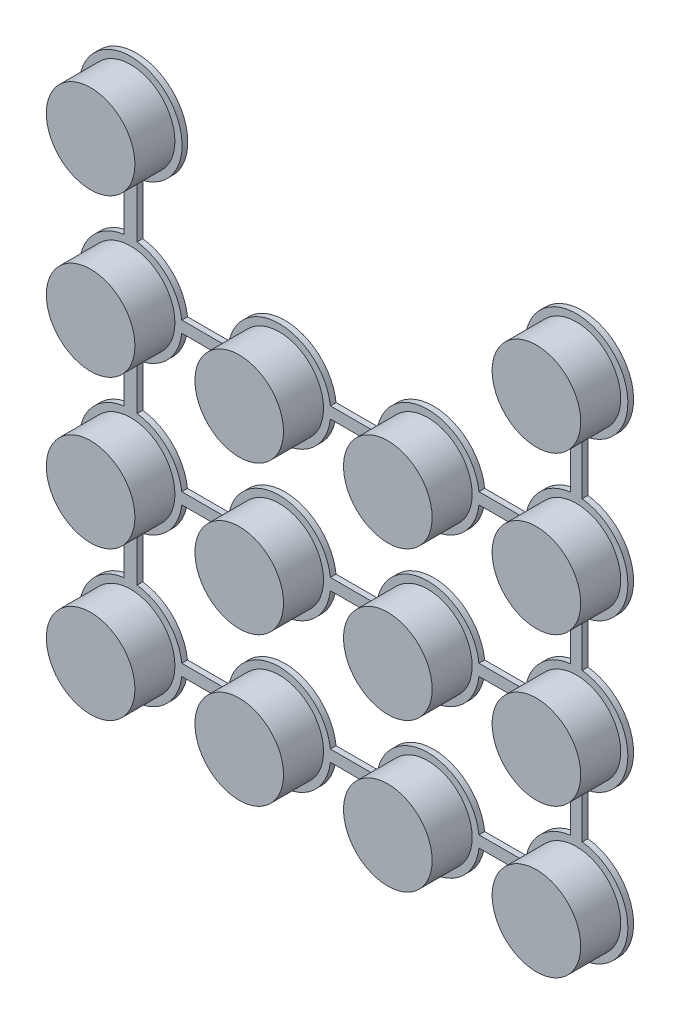
from build123d import *

# Parameters (mm, degrees)
BOSS_EXTRUDE1_DEPTH = 1
SKETCH2_R           = 7.75
BOSS_EXTRUDE2_DEPTH = 7


with BuildPart() as part:
    # Sketch1 → Boss-Extrude1 (new body)
    with BuildSketch(Plane.XY):
        with BuildLine():
            Line((-40.125, 93.570589325), (-40.125, 83.929410675))
            ThreePointArc((-40.125, 83.929410675), (-48, 75), (-40.125, 66.070589325))
            Line((-40.125, 66.070589325), (-40.125, 57.929410675))
            ThreePointArc((-40.125, 57.929410675), (-48, 49), (-40.125, 40.070589325))
            Line((-40.125, 40.070589325), (-40.125, 31.929410675))
            ThreePointArc((-40.125, 31.929410675), (-45.319299992, 16.591689176), (-30.05572809, 22))
            Line((-30.05572809, 22), (-21.94427191, 22))
            ThreePointArc((-21.94427191, 22), (-13, 14), (-4.05572809, 22))
            Line((-4.05572809, 22), (4.05572809, 22))
            ThreePointArc((4.05572809, 22), (13, 14), (21.94427191, 22))
            Line((21.94427191, 22), (30.05572809, 22))
            ThreePointArc((30.05572809, 22), (45.363961031, 16.636038969), (40, 31.94427191))
            Line((40, 31.94427191), (40, 40.05572809))
            ThreePointArc((40, 40.05572809), (48, 49), (40, 57.94427191))
            Line((40, 57.94427191), (40, 66.05572809))
            ThreePointArc((40, 66.05572809), (48, 75), (40, 83.94427191))
            Line((40, 83.94427191), (40, 93.55572809))
            ThreePointArc((40, 93.55572809), (39, 111.5), (38, 93.55572809))
            Line((38, 93.55572809), (38, 83.94427191))
            ThreePointArc((38, 83.94427191), (32.636038969, 81.363961031), (30.05572809, 76))
            Line((30.05572809, 76), (21.94427191, 76))
            ThreePointArc((21.94427191, 76), (13, 84), (4.05572809, 76))
            Line((4.05572809, 76), (-4.05572809, 76))
            ThreePointArc((-4.05572809, 76), (-13, 84), (-21.94427191, 76))
            Line((-21.94427191, 76), (-30.05572809, 76))
            ThreePointArc((-30.05572809, 76), (-32.591689176, 81.319299992), (-37.875, 83.929410675))
            Line((-37.875, 83.929410675), (-37.875, 93.570589325))
            ThreePointArc((-37.875, 93.570589325), (-39, 111.5), (-40.125, 93.570589325))
        make_face()
        with BuildLine():
            Line((-30.05572809, 74), (-21.94427191, 74))
            ThreePointArc((-21.94427191, 74), (-13, 66), (-4.05572809, 74))
            Line((-4.05572809, 74), (4.05572809, 74))
            ThreePointArc((4.05572809, 74), (13, 66), (21.94427191, 74))
            Line((21.94427191, 74), (30.05572809, 74))
            ThreePointArc((30.05572809, 74), (32.636038969, 68.636038969), (38, 66.05572809))
            Line((38, 66.05572809), (38, 57.94427191))
            ThreePointArc((38, 57.94427191), (32.636038969, 55.363961031), (30.05572809, 50))
            Line((30.05572809, 50), (21.94427191, 50))
            ThreePointArc((21.94427191, 50), (13, 58), (4.05572809, 50))
            Line((4.05572809, 50), (-4.05572809, 50))
            ThreePointArc((-4.05572809, 50), (-13, 58), (-21.94427191, 50))
            Line((-21.94427191, 50), (-30.05572809, 50))
            ThreePointArc((-30.05572809, 50), (-32.591689176, 55.319299992), (-37.875, 57.929410675))
            Line((-37.875, 57.929410675), (-37.875, 66.070589325))
            ThreePointArc((-37.875, 66.070589325), (-32.591689176, 68.680700008), (-30.05572809, 74))
        make_face(mode=Mode.SUBTRACT)
        with BuildLine():
            Line((-30.05572809, 48), (-21.94427191, 48))
            ThreePointArc((-21.94427191, 48), (-13, 40), (-4.05572809, 48))
            Line((-4.05572809, 48), (4.05572809, 48))
            ThreePointArc((4.05572809, 48), (13, 40), (21.94427191, 48))
            Line((21.94427191, 48), (30.05572809, 48))
            ThreePointArc((30.05572809, 48), (32.636038969, 42.636038969), (38, 40.05572809))
            Line((38, 40.05572809), (38, 31.94427191))
            ThreePointArc((38, 31.94427191), (32.636038969, 29.363961031), (30.05572809, 24))
            Line((30.05572809, 24), (21.94427191, 24))
            ThreePointArc((21.94427191, 24), (13, 32), (4.05572809, 24))
            Line((4.05572809, 24), (-4.05572809, 24))
            ThreePointArc((-4.05572809, 24), (-13, 32), (-21.94427191, 24))
            Line((-21.94427191, 24), (-30.05572809, 24))
            ThreePointArc((-30.05572809, 24), (-32.591689176, 29.319299992), (-37.875, 31.929410675))
            Line((-37.875, 31.929410675), (-37.875, 40.070589325))
            ThreePointArc((-37.875, 40.070589325), (-32.591689176, 42.680700008), (-30.05572809, 48))
        make_face(mode=Mode.SUBTRACT)
    extrude(amount=BOSS_EXTRUDE1_DEPTH)

    # Sketch2 → Boss-Extrude2 (add)
    with BuildSketch(Plane.XY.offset(1)):
        with Locations((-39, 102.5)):
            Circle(SKETCH2_R)
        with Locations((-39, 75)):
            Circle(SKETCH2_R)
        with Locations((-39, 49)):
            Circle(SKETCH2_R)
        with Locations((-39, 23)):
            Circle(SKETCH2_R)
        with Locations((-13, 75)):
            Circle(SKETCH2_R)
        with Locations((-13, 49)):
            Circle(SKETCH2_R)
        with Locations((-13, 23)):
            Circle(SKETCH2_R)
        with Locations((13, 75)):
            Circle(SKETCH2_R)
        with Locations((39, 102.5)):
            Circle(SKETCH2_R)
        with Locations((39, 23)):
            Circle(SKETCH2_R)
        with Locations((13, 23)):
            Circle(SKETCH2_R)
        with Locations((39, 49)):
            Circle(SKETCH2_R)
        with Locations((13, 49)):
            Circle(SKETCH2_R)
        with Locations((39, 75)):
            Circle(SKETCH2_R)
    extrude(amount=BOSS_EXTRUDE2_DEPTH)


solid = part.part
